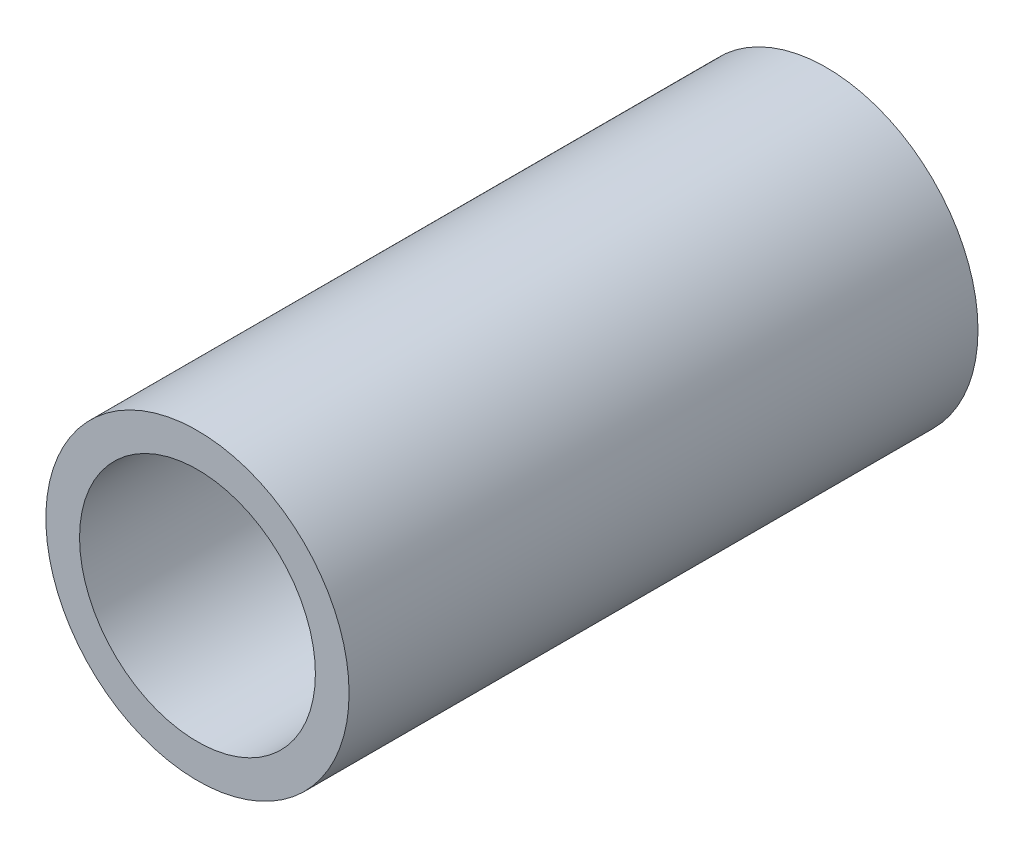
from build123d import *

# Parameters (mm, degrees)
SKETCH1_R           = 13.5
SKETCH1_R_2         = 10.5
BOSS_EXTRUDE1_DEPTH = 28


with BuildPart() as part:
    # Sketch1 → Boss-Extrude1 (new, symmetric)
    with BuildSketch(Plane.XY):
        Circle(SKETCH1_R)
        Circle(SKETCH1_R_2, mode=Mode.SUBTRACT)
    extrude(amount=BOSS_EXTRUDE1_DEPTH, both=True)


solid = part.part
